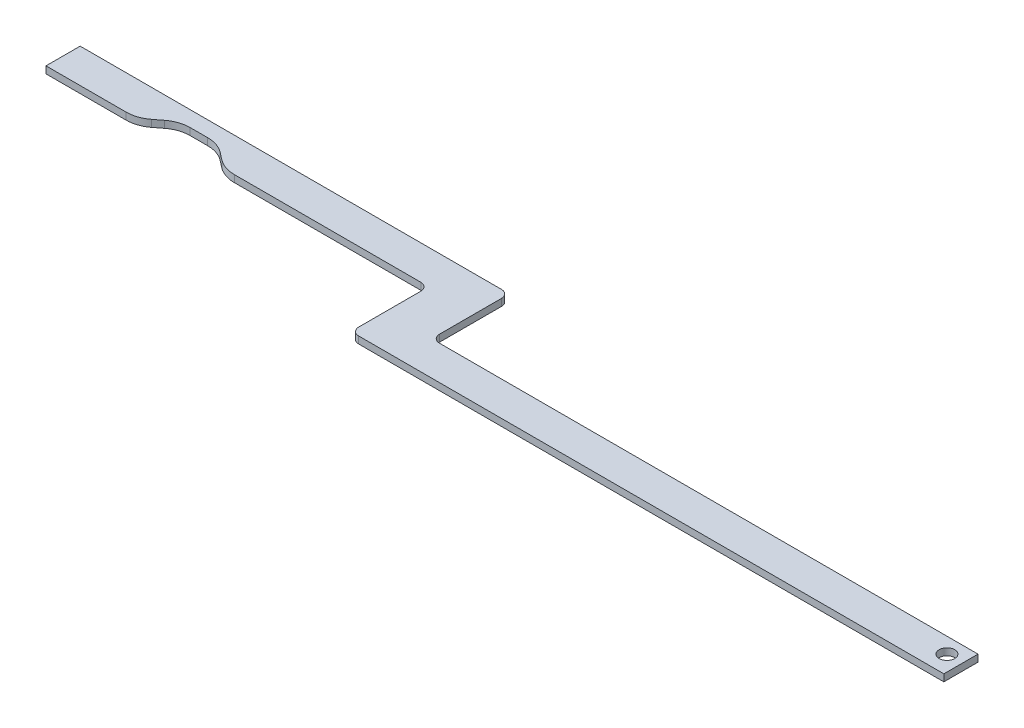
SolidWorks part; units mm, degrees
ref_plane "Front Plane" through (0, 0, 0) normal (0, 0, 1) x (1, 0, 0)
ref_plane "Top Plane" through (0, 0, 0) normal (0, 1, 0) x (1, 0, 0)
ref_plane "Right Plane" through (0, 0, 0) normal (1, 0, 0) x (0, 0, -1)
sketch "Sketch1" plane through (0, 0, 0) normal (0, 1, 0) x (1, 0, 0)
  line L0 (0, 0) -> (271.5, 0)
  line L1 (276.5, -5) -> (276.5, -45)
  line L2 (281.5, -50) -> (628.5, -50)
  line L3 (628.5, -50) -> (628.5, -72)
  line L4 (628.5, -72) -> (251.5, -72)
  line L5 (246.5, -67) -> (246.5, -27)
  line L6 (241.5, -22) -> (121.3372, -22)
  line L7 (0, -22) -> (0, 0)
  line L8 (51.6628, -22) -> (0, -22)
  line L9 (68.5937, -14.1855) -> (63.9063, -17.8145)
  line L10 (80.8372, -10) -> (92.1628, -10)
  line L11 (104.4063, -14.1855) -> (109.0937, -17.8145)
  arc A0 (121.3372, -22) -> (109.0937, -17.8145) centre (121.3372, -2) cw
  circle A1 centre (618.5, -60) radius 5
  arc A2 (63.9063, -17.8145) -> (51.6628, -22) centre (51.6628, -2) cw
  arc A3 (68.5937, -14.1855) -> (80.8372, -10) centre (80.8372, -30) cw
  arc A4 (92.1628, -10) -> (104.4063, -14.1855) centre (92.1628, -30) cw
  arc A5 (246.5, -27) -> (241.5, -22) centre (241.5, -27) ccw
  arc A6 (251.5, -72) -> (246.5, -67) centre (251.5, -67) cw
  arc A7 (276.5, -45) -> (281.5, -50) centre (281.5, -45) ccw
  arc A8 (271.5, 0) -> (276.5, -5) centre (271.5, -5) cw
  point P16 (114.5, -22)
  point P20 (58.5, -22)
  point P23 (74, -10)
  point P26 (99, -10)
  point P29 (246.5, -22)
  point P32 (246.5, -72)
  dimension "D7" = 10
  dimension "D8" = 12
  dimension "D9" = 10
  dimension "D15" = 20
  dimension "D16" = 5
  dimension "D1" = 628.5
  dimension "D2" = 22
  dimension "D3" = 50
  dimension "D4" = 352
  dimension "D5" = 382
  dimension "D6" = 72
  dimension "D10" = 514
  dimension "D11" = 25
  dimension "D12" = 15.5
  dimension "D13" = 12
  dimension "D14" = 56
extrude "Boss-Extrude1" add sketch "Sketch1" along normal blind 4.5
